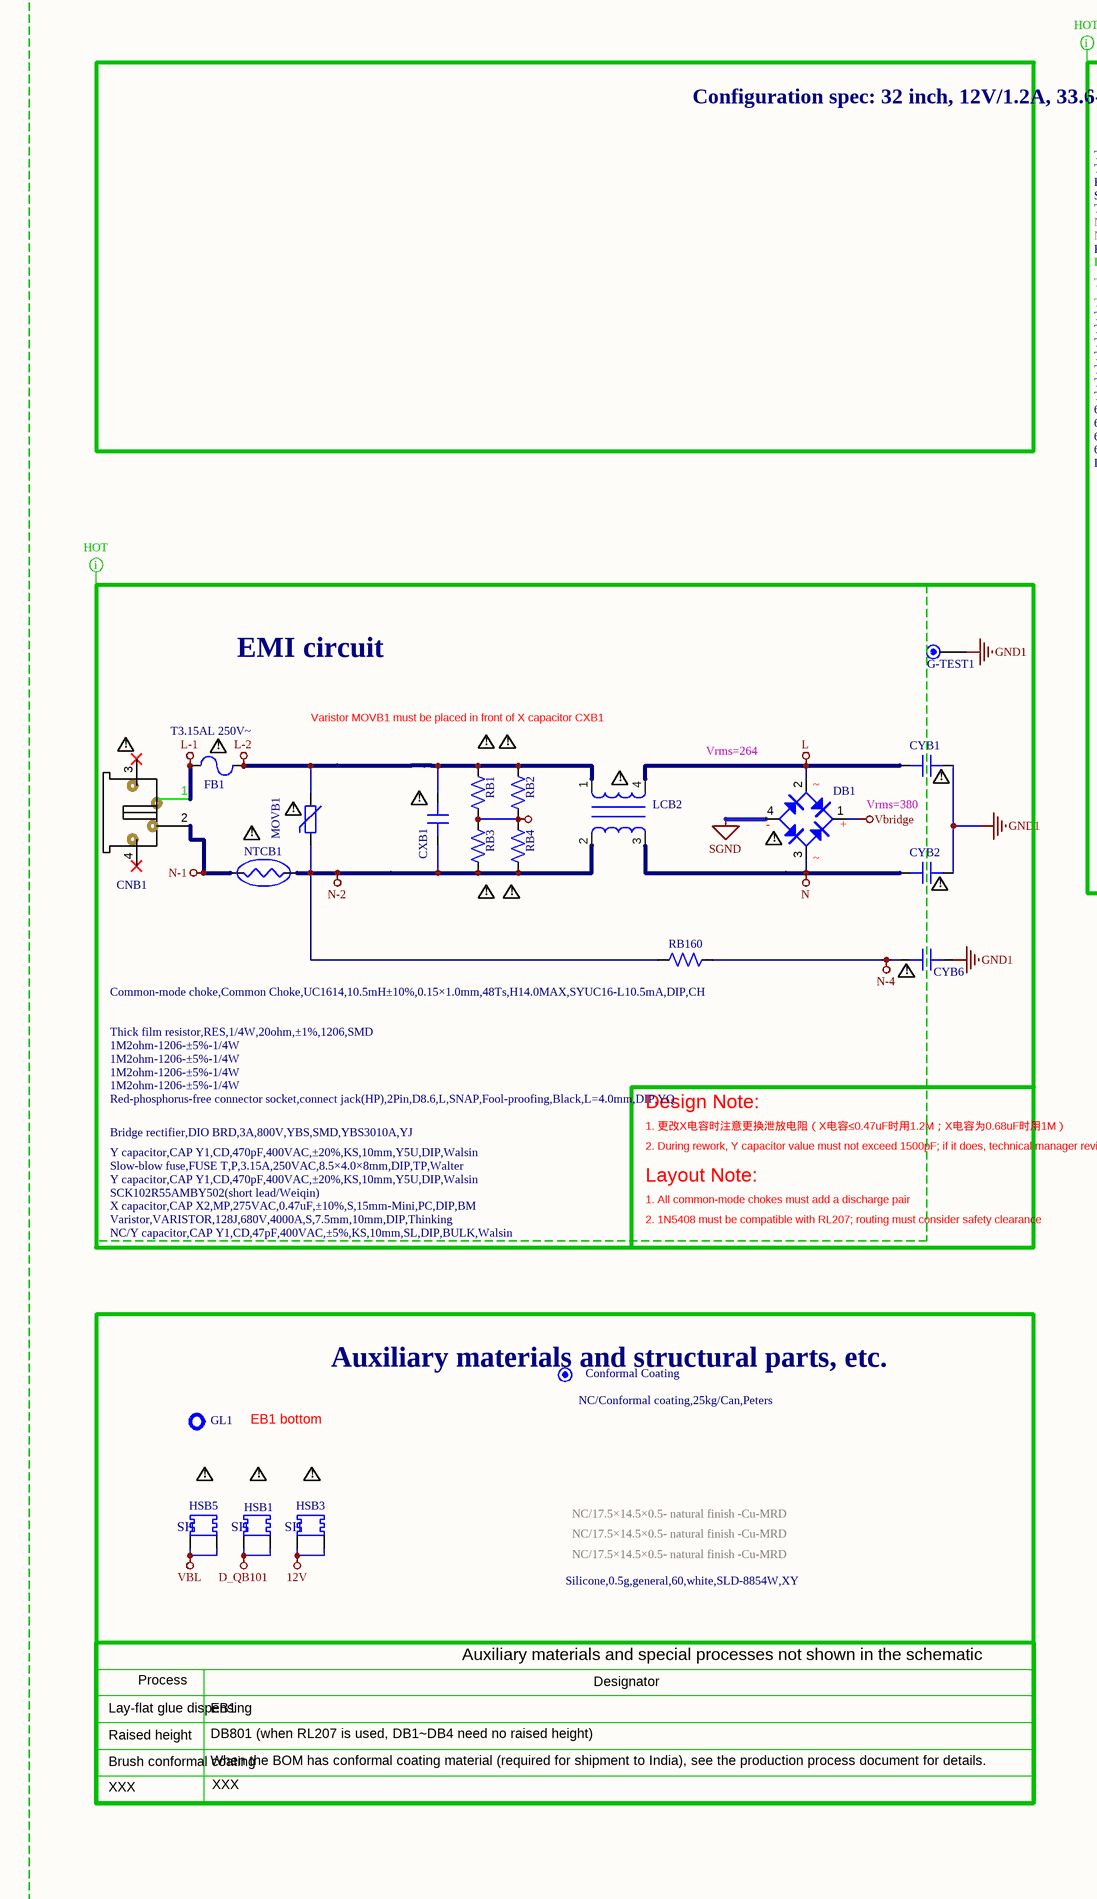
[diagram p0: MISC86383-5.SchDoc, left]
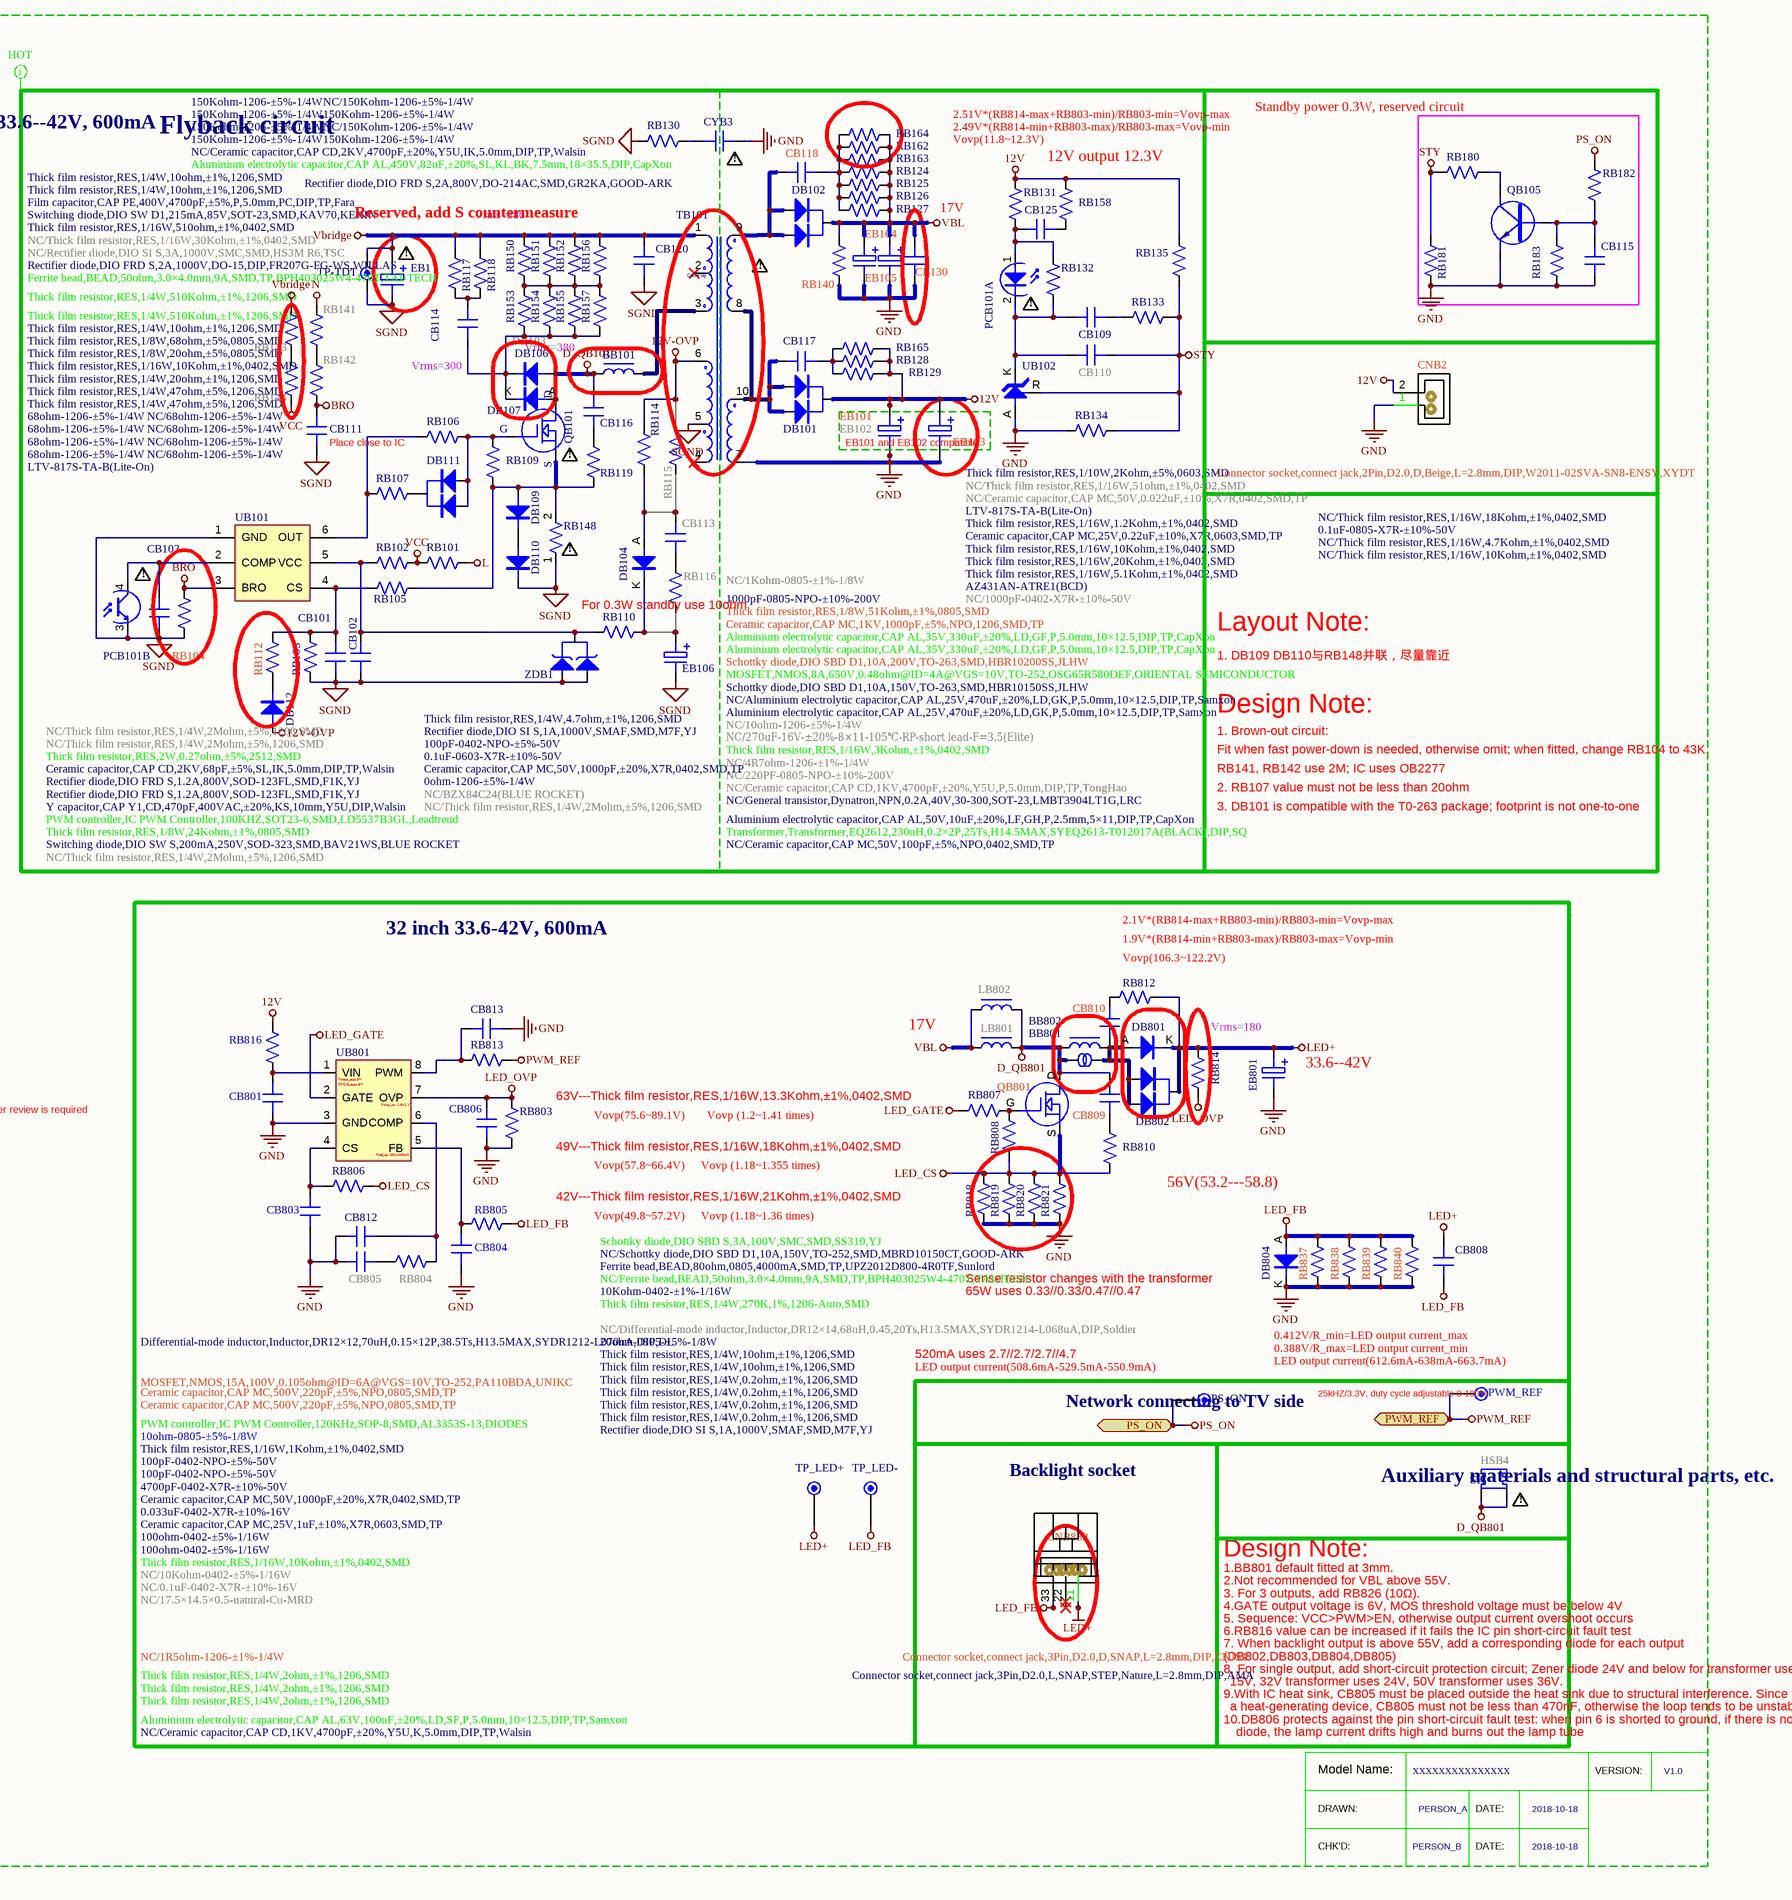
[diagram p1: MISC86383-5.SchDoc, right]
# Altium project MISC86383-33.PrjPCB (part 7 of 8)

## Sheet MISC86383-5.SchDoc: MISC86383
size A2

### Parts
BB101  Ferrite bead,BEAD,50ohm,3.0×4.0mm,9A,SMD,TP,BPH403025W4-470T,TAI-TECH  [L(4*3*2.55)-S]
BB801  Ferrite bead,BEAD,80ohm,0805,4000mA,SMD,TP,UPZ2012D800-4R0TF,Sunlord  [R0805]
BB802  NC/Ferrite bead,BEAD,50ohm,3.0×4.0mm,9A,SMD,TP,BPH403025W4-470T,TAI-TECH  [L(4*3*2.55)-S]
CB101  100pF-0402-NPO-±5%-50V  [C0402]
CB102  0.1uF-0603-X7R-±10%-50V  [C0603]
CB103  Ceramic capacitor,CAP MC,50V,1000pF,±20%,X7R,0402,SMD,TP  [C0402]
CB109  Ceramic capacitor,CAP MC,25V,0.22uF,±10%,X7R,0603,SMD,TP  [C0603]
CB110  NC/1000pF-0402-X7R-±10%-50V  [C0402]
CB111  NC/Ceramic capacitor,CAP MC,50V,100pF,±5%,NPO,0402,SMD,TP  [C0402]
CB113  NC/220PF-0805-NPO-±10%-200V  [C0805]
CB114  Film capacitor,CAP PE,400V,4700pF,±5%,P,5.0mm,PC,DIP,TP,Fara  [CAP8*2.5-V-5]
CB115  0.1uF-0805-X7R-±10%-50V  [C0805]
CB116  Ceramic capacitor,CAP CD,2KV,68pF,±5%,SL,IK,5.0mm,DIP,TP,Walsin  [CAP6.5*5-V-5-1]
CB117  1000pF-0805-NPO-±10%-200V  [C0805]
CB118  Ceramic capacitor,CAP MC,1KV,1000pF,±5%,NPO,1206,SMD,TP  [C1206]
CB120  NC/Ceramic capacitor,CAP CD,2KV,4700pF,±20%,Y5U,IK,5.0mm,DIP,TP,Walsin  [CAP10*4.5-V-5]
CB125  NC/Ceramic capacitor,CAP MC,50V,0.022uF,±10%,X7R,0402,SMD,TP  [C0402]
CB130  NC/Ceramic capacitor,CAP CD,1KV,4700pF,±20%,Y5U,P,5.0mm,DIP,TP,TongHao  [CAP9.8*4-V-5]
CB801  Ceramic capacitor,CAP MC,25V,1uF,±10%,X7R,0603,SMD,TP  [C0603]
CB803  100pF-0402-NPO-±5%-50V  [C0402]
CB804  4700pF-0402-X7R-±10%-50V  [C0402]
CB805  NC/0.1uF-0402-X7R-±10%-16V  [C0402]
CB806  Ceramic capacitor,CAP MC,50V,1000pF,±20%,X7R,0402,SMD,TP  [C0402]
CB808  NC/Ceramic capacitor,CAP CD,1KV,4700pF,±20%,Y5U,K,5.0mm,DIP,TP,Walsin  [CAP10*4.5-V-5]
CB809  Ceramic capacitor,CAP MC,500V,220pF,±5%,NPO,0805,SMD,TP  [C0805]
CB810  Ceramic capacitor,CAP MC,500V,220pF,±5%,NPO,0805,SMD,TP  [C0805]
CB812  0.033uF-0402-X7R-±10%-16V  [C0402]
CB813  100pF-0402-NPO-±5%-50V  [C0402]
CNB1  Red-phosphorus-free connector socket,connect jack(HP),2Pin,D8.6,L,SNAP,Fool-proofing,Black,L=4.0mm,DIP,YQ  [CON2-H8.6-1]
CNB2  Connector socket,connect jack,2Pin,D2.0,D,Beige,L=2.8mm,DIP,W2011-02SVA-SN8-ENSY,XYDT  [SIP2/2.0D-1]
CNB832  Connector socket,connect jack,3Pin,D2.0,D,SNAP,L=2.8mm,DIP,CNJST  [SIP3/2.0D-CP]
CNB833  Connector socket,connect jack,3Pin,D2.0,L,SNAP,STEP,Nature,L=2.8mm,DIP,AMA  [SIP3H/2.0D-3]
Conformal_Coating  NC/Conformal coating,25kg/Can,Peters  [Conformal Coating]
CXB1  X capacitor,CAP X2,MP,275VAC,0.47uF,±10%,S,15mm-Mini,PC,DIP,BM  [CAP18*8.5-V-15]
CYB1  Y capacitor,CAP Y1,CD,470pF,400VAC,±20%,KS,10mm,Y5U,DIP,Walsin  [CAP13*5-V-10-1]
CYB2  Y capacitor,CAP Y1,CD,470pF,400VAC,±20%,KS,10mm,Y5U,DIP,Walsin  [CAP13*5-V-10-1]
CYB3  Y capacitor,CAP Y1,CD,470pF,400VAC,±20%,KS,10mm,Y5U,DIP,Walsin  [CAP13*5-V-10-1]
CYB6  NC/Y capacitor,CAP Y1,CD,47pF,400VAC,±5%,KS,10mm,SL,DIP,BULK,Walsin  [CAP13*5-V-10-1]
DB1  Bridge rectifier,DIO BRD,3A,800V,YBS,SMD,YBS3010A,YJ  [B/YBS3010A]
DB101  Schottky diode,DIO SBD D1,10A,150V,TO-263,SMD,HBR10150SS,JLHW  [D2PAK3]
DB102  Schottky diode,DIO SBD D1,10A,200V,TO-263,SMD,HBR10200SS,JLHW  [D2PAK3]
DB103  NC/Rectifier diode,DIO SI S,3A,1000V,SMC,SMD,HS3M R6,TSC  [DIODE-SMC]
DB104  Rectifier diode,DIO SI S,1A,1000V,SMAF,SMD,M7F,YJ  [DIODE-S-2]
DB106  Rectifier diode,DIO FRD S,2A,1000V,DO-15,DIP,FR207G-FG-WS,WILLAS  [D2-H-15]
DB107  Rectifier diode,DIO FRD S,2A,800V,DO-214AC,SMD,GR2KA,GOOD-ARK  [DIODE-S-2]
DB109  Rectifier diode,DIO FRD S,1.2A,800V,SOD-123FL,SMD,F1K,YJ  [DIODE-S-14]
DB110  Rectifier diode,DIO FRD S,1.2A,800V,SOD-123FL,SMD,F1K,YJ  [DIODE-S-14]
DB111  Switching diode,DIO SW D1,215mA,85V,SOT-23,SMD,KAV70,KEXIN  [SO-23]
DB112  Switching diode,DIO SW S,200mA,250V,SOD-323,SMD,BAV21WS,BLUE ROCKET  [DIODE-S-12]
DB801  Schottky diode,DIO SBD S,3A,100V,SMC,SMD,SS310,YJ  [DIODE-SMC]
DB802  NC/Schottky diode,DIO SBD D1,10A,150V,TO-252,SMD,MBRD10150CT,GOOD-ARK  [TO-252]
DB804  Rectifier diode,DIO SI S,1A,1000V,SMAF,SMD,M7F,YJ  [DIODE-S-2]
EB1  Aluminium electrolytic capacitor,CAP AL,450V,82uF,±20%,SL,KL,BK,7.5mm,18×35.5,DIP,CapXon  [EC(18*36)-H7.5-1]
EB101  Aluminium electrolytic capacitor,CAP AL,25V,470uF,±20%,LD,GK,P,5.0mm,10×12.5,DIP,TP,Samxon  [EC(10*12.5)-V-5]
EB102  NC/270uF-16V-±20%-8×11-105℃-RP-short lead-F=3.5(Elite)  [EC(8*11)-V-3.5]
EB103  NC/Aluminium electrolytic capacitor,CAP AL,25V,470uF,±20%,LD,GK,P,5.0mm,10×12.5,DIP,TP,Samxon  [EC(10*12.5)-V-5]
EB104  Aluminium electrolytic capacitor,CAP AL,35V,330uF,±20%,LD,GF,P,5.0mm,10×12.5,DIP,TP,CapXon  [EC(10*12.5)-V-5]
EB105  Aluminium electrolytic capacitor,CAP AL,35V,330uF,±20%,LD,GF,P,5.0mm,10×12.5,DIP,TP,CapXon  [EC(10*12.5)-V-5]
EB106  Aluminium electrolytic capacitor,CAP AL,50V,10uF,±20%,LF,GH,P,2.5mm,5×11,DIP,TP,CapXon  [EC(5*11)-V-2.5]
EB801  Aluminium electrolytic capacitor,CAP AL,63V,100uF,±20%,LD,SF,P,5.0mm,10×12.5,DIP,TP,Samxon  [EC(10*12.5)-V-5]
FB1  Slow-blow fuse,FUSE T,P,3.15A,250VAC,8.5×4.0×8mm,DIP,TP,Walter  [FUSE8.5*4-V-5(T3.15AL 250V~)]
G-TEST1  TEST  [TP]  (value not drawn)
GL1  Silicone,0.5g,general,60,white,SLD-8854W,XY  [Silica gel-20]
HSB1  NC/17.5×14.5×0.5- natural finish -Cu-MRD  [HS038]
HSB3  NC/17.5×14.5×0.5- natural finish -Cu-MRD  [HS038]
HSB4  NC/17.5×14.5×0.5-natural-Cu-MRD  [HS038]
HSB5  NC/17.5×14.5×0.5- natural finish -Cu-MRD  [HS038]
LB801  Differential-mode inductor,Inductor,DR12×12,70uH,0.15×12P,38.5Ts,H13.5MAX,SYDR1212-L070uA,DIP,DL  [L/LC2/15*14.5-V7.5]
LB802  NC/Differential-mode inductor,Inductor,DR12×14,68uH,0.45,20Ts,H13.5MAX,SYDR1214-L068uA,DIP,Soldier  [L(13.5*15.5)-V-5]
LCB2  Common-mode choke,Common Choke,UC1614,10.5mH±10%,0.15×1.0mm,48Ts,H14.0MAX,SYUC16-L10.5mA,DIP,CH  [L/LC4/21*17-H-17*13]
MOVB1  Varistor,VARISTOR,128J,680V,4000A,S,7.5mm,10mm,DIP,Thinking  [VR(13*5)-V-7.5]
NTCB1  SCK102R55AMBY502(short lead/Weiqin)  [NTC(10*5)-V5]
PCB101  LTV-817S-TA-B(Lite-On)  [OC4-S-1]  (parts A,B of 2)
PS_ON  TEST  [TP_BL]  (value not drawn)
PWM_REF  NC/TEST  [TP_BL]  (value not drawn)
QB101  MOSFET,NMOS,8A,650V,0.48ohm@ID=4A@VGS=10V,TO-252,OSG65R580DEF,ORIENTAL SEMICONDUCTOR  [D2PAK3]
QB105  NC/General transistor,Dynatron,NPN,0.2A,40V,30-300,SOT-23,LMBT3904LT1G,LRC  [SOT-23]
QB801  MOSFET,NMOS,15A,100V,0.105ohm@ID=6A@VGS=10V,TO-252,PA110BDA,UNIKC  [TO-252-GDS]
RB1  1M2ohm-1206-±5%-1/4W  [R1206]
RB2  1M2ohm-1206-±5%-1/4W  [R1206]
RB3  1M2ohm-1206-±5%-1/4W  [R1206]
RB4  1M2ohm-1206-±5%-1/4W  [R1206]
RB101  Thick film resistor,RES,1/4W,510Kohm,±1%,1206,SMD  [R1206]
RB102  Thick film resistor,RES,1/4W,510Kohm,±1%,1206,SMD  [R1206]
RB103  Thick film resistor,RES,1/16W,3Kohm,±1%,0402,SMD  [R0402]
RB104  NC/Thick film resistor,RES,1/16W,30Kohm,±1%,0402,SMD  [R0402]
RB105  Thick film resistor,RES,1/16W,510ohm,±1%,0402,SMD  [R0402]
RB106  Thick film resistor,RES,1/8W,68ohm,±5%,0805,SMD  [R0805]
RB107  Thick film resistor,RES,1/8W,20ohm,±5%,0805,SMD  [R0805]
RB109  Thick film resistor,RES,1/16W,10Kohm,±1%,0402,SMD  [R0402]
RB110  0ohm-1206-±5%-1/4W  [R1206]
RB112  Thick film resistor,RES,1/8W,24Kohm,±1%,0805,SMD  [R0805]
RB114  Thick film resistor,RES,1/4W,4.7ohm,±1%,1206,SMD  [R1206]
RB115  NC/4R7ohm-1206-±1%-1/4W  [R1206]
RB116  NC/10ohm-1206-±5%-1/4W  [R1206]
RB117  Thick film resistor,RES,1/4W,10ohm,±1%,1206,SMD  [R1206]
RB118  Thick film resistor,RES,1/4W,10ohm,±1%,1206,SMD  [R1206]
RB119  Thick film resistor,RES,1/4W,10ohm,±1%,1206,SMD  [R1206]
RB124  68ohm-1206-±5%-1/4W  [R1206]
RB125  68ohm-1206-±5%-1/4W  [R1206]
RB126  68ohm-1206-±5%-1/4W  [R1206]
RB127  68ohm-1206-±5%-1/4W  [R1206]
RB128  Thick film resistor,RES,1/4W,47ohm,±5%,1206,SMD  [R1206]
RB129  Thick film resistor,RES,1/4W,47ohm,±5%,1206,SMD  [R1206]
RB130  Thick film resistor,RES,1/4W,20ohm,±1%,1206,SMD  [R1206]
RB131  Thick film resistor,RES,1/10W,2Kohm,±5%,0603,SMD  [R0603]
RB132  Thick film resistor,RES,1/16W,1.2Kohm,±1%,0402,SMD  [R0402]
RB133  Thick film resistor,RES,1/16W,10Kohm,±1%,0402,SMD  [R0402]
RB134  Thick film resistor,RES,1/16W,5.1Kohm,±1%,0402,SMD  [R0402]
RB135  Thick film resistor,RES,1/16W,20Kohm,±1%,0402,SMD  [R0402]
RB140  Thick film resistor,RES,1/8W,51Kohm,±1%,0805,SMD  [R0805]
RB141  NC/Thick film resistor,RES,1/4W,2Mohm,±5%,1206,SMD  [R1206]
RB142  NC/Thick film resistor,RES,1/4W,2Mohm,±5%,1206,SMD  [R1206]
RB143  NC/Thick film resistor,RES,1/4W,2Mohm,±5%,1206,SMD  [R1206]
RB144  NC/Thick film resistor,RES,1/4W,2Mohm,±5%,1206,SMD  [R1206]
RB148  Thick film resistor,RES,2W,0.27ohm,±5%,2512,SMD  [R2512-1]
RB150  150Kohm-1206-±5%-1/4W  [R1206]
RB151  150Kohm-1206-±5%-1/4W  [R1206]
RB152  150Kohm-1206-±5%-1/4W  [R1206]
RB153  150Kohm-1206-±5%-1/4W  [R1206]
RB154  150Kohm-1206-±5%-1/4W  [R1206]
RB155  150Kohm-1206-±5%-1/4W  [R1206]
RB156  NC/150Kohm-1206-±5%-1/4W  [R1206]
RB157  NC/150Kohm-1206-±5%-1/4W  [R1206]
RB158  NC/Thick film resistor,RES,1/16W,51ohm,±1%,0402,SMD  [R0402]
RB160  Thick film resistor,RES,1/4W,20ohm,±1%,1206,SMD  [R1206]
RB162  NC/68ohm-1206-±5%-1/4W  [R1206]
RB163  NC/68ohm-1206-±5%-1/4W  [R1206]
RB164  NC/68ohm-1206-±5%-1/4W  [R1206]
RB165  NC/68ohm-1206-±5%-1/4W  [R1206]
RB180  NC/Thick film resistor,RES,1/16W,18Kohm,±1%,0402,SMD  [R0402]
RB181  NC/1Kohm-0805-±1%-1/8W  [R0805]
RB182  NC/Thick film resistor,RES,1/16W,4.7Kohm,±1%,0402,SMD  [R0402]
RB183  NC/Thick film resistor,RES,1/16W,10Kohm,±1%,0402,SMD  [R0402]
RB803  Thick film resistor,RES,1/16W,10Kohm,±1%,0402,SMD  [R0402]
RB804  NC/10Kohm-0402-±5%-1/16W  [R0402]
RB805  100ohm-0402-±5%-1/16W  [R0402]
RB806  Thick film resistor,RES,1/16W,1Kohm,±1%,0402,SMD  [R0402]
RB807  20ohm-0805-±5%-1/8W  [R0805]
RB808  10Kohm-0402-±1%-1/16W  [R0402]
RB810  Thick film resistor,RES,1/4W,10ohm,±1%,1206,SMD  [R1206]
RB812  Thick film resistor,RES,1/4W,10ohm,±1%,1206,SMD  [R1206]
RB813  100ohm-0402-±5%-1/16W  [R0402]
RB814  Thick film resistor,RES,1/4W,270K,1%,1206-Auto,SMD  [R1206]
RB816  10ohm-0805-±5%-1/8W  [R0805]
RB818  Thick film resistor,RES,1/4W,0.2ohm,±1%,1206,SMD  [R1206]
RB819  Thick film resistor,RES,1/4W,0.2ohm,±1%,1206,SMD  [R1206]
RB820  Thick film resistor,RES,1/4W,0.2ohm,±1%,1206,SMD  [R1206]
RB821  Thick film resistor,RES,1/4W,0.2ohm,±1%,1206,SMD  [R1206]
RB837  Thick film resistor,RES,1/4W,2ohm,±1%,1206,SMD  [R1206]
RB838  Thick film resistor,RES,1/4W,2ohm,±1%,1206,SMD  [R1206]
RB839  Thick film resistor,RES,1/4W,2ohm,±1%,1206,SMD  [R1206]
RB840  NC/1R5ohm-1206-±1%-1/4W  [R1206]
TB101  Transformer,Transformer,EQ2612,230uH,0.2×2P,25Ts,H14.5MAX,SYEQ2613-T012017A(BLACK),DIP,SQ  [T/EQ2612*10]
TP-TDT  NC/  [TP-TDT]  (value not drawn)
TP_LED+  NC/  [TP]  (value not drawn)
TP_LED-  NC/  [TP]  (value not drawn)
UB101  PWM controller,IC PWM Controller,100KHZ,SOT23-6,SMD,LD5537B3GL,Leadtrend  [SOT-26]
UB102  AZ431AN-ATRE1(BCD)  [SOT-23-RAK]
UB801  PWM controller,IC PWM Controller,120KHz,SOP-8,SMD,AL3353S-13,DIODES  [SO-8A]
ZDB1  NC/BZX84C24(BLUE ROCKET)  [SO-23]

### Blocks framed on the sheet
Vrms=380: DB103 DB106 DB107
EB101 and EB102 compatible: EB101-EB103
EMI circuit: CNB1 CXB1 CYB1 CYB2 CYB6 DB1 FB1 G-TEST1 LCB2 MOVB1 NTCB1 RB1-RB4 RB160
Auxiliary materials and structural parts, etc.: Conformal_Coating GL1 HSB1 HSB3 HSB5

### Ports
PS_ON, PWM_REF

### Nets
12V: CNB2.2 DB101.2 EB101.1 EB102.1 EB103.1 HSB3.1 HSB3.2 RB128.2 RB129.2 RB131.2 RB135.1 RB158.2 RB165.2 RB816.1
12V-OVP: DB112.A RB114.2 RB115.2 TB101.6
BRO: CB111.1 RB104.2 RB142.1 UB101.3(BRO)
D_QB101: BB101.1 CB116.2 DB103.A DB106.A DB107.A HSB1.1 HSB1.2 QB101.2(D)
D_QB801: BB801.1 BB802.1 CB809.2 HSB4.1 HSB4.2 LB801.2 LB802.2 QB801.D
GND: CB115.2 CB130.1 CB801.1 CB803.2 CB804.2 CB805.1 CB806.2 CB812.1 CB813.1 CNB2.1 CYB3.2 DB804.K EB101.2 EB102.2 EB103.2 EB104.2 EB105.2 EB801.2 QB105.E RB134.1 RB140.2 RB181.1 RB183.2 RB803.1 RB818.2 RB819.2 RB820.2 RB821.2 RB837.1 RB838.1 RB839.2 RB840.1 TB101.7 UB102.A UB801.3(GND)
GND1: CYB1.2 CYB2.2 CYB6.2 G-TEST1.1
L: CYB1.1 DB1.2 LCB2.4 RB101.1
L-1: CNB1.1 FB1.1
L-2: CXB1.1 FB1.2 LCB2.1 MOVB1.1 RB1.1 RB2.1
L-N: RB1.2 RB2.2 RB3.1 RB4.1
LED+: CB808.2 CNB832.1 CNB833.1 DB801.K DB802.2 EB801.1 RB812.2 RB814.1 TP_LED+.1
LED_CS: QB801.S RB806.2 RB808.1 RB810.2 RB818.1 RB819.1 RB820.1 RB821.1
LED_FB: CB808.1 CNB832.3 CNB833.3 DB804.A RB805.2 RB837.2 RB838.2 RB839.1 RB840.2 TP_LED-.1
LED_GATE: RB807.1 UB801.2(GATE)
LED_OVP: CB806.1 RB803.2 RB814.2 UB801.7(OVP)
N: CYB2.1 DB1.3 LCB2.3 RB141.2
N-1: CNB1.2 NTCB1.2
N-2: CXB1.2 LCB2.2 MOVB1.2 NTCB1.1 RB3.2 RB4.2 RB160.1
N-4: CYB6.1 RB160.2
PS_ON: PS_ON.1 RB182.2 ; port PS_ON
PWM_REF: PWM_REF.1 RB813.2 ; port PWM_REF
SGND: CB101.2 CB102.2 CB103.2 CB111.2 CB120.1 DB1.4 DB110.K EB1.2 EB106.2 PCB101.3 RB103.1 RB104.1 RB130.1 RB148.1 TB101.5 TP-TDT.2 UB101.1(GND) ZDB1.1 ZDB1.3
STY: CB110.2 RB133.1 RB134.2 RB135.2 RB180.2 RB181.2 UB102.R
VBL: CB130.2 DB102.2 EB104.1 EB105.1 HSB5.1 HSB5.2 LB801.1 LB802.1 RB124.2 RB125.2 RB126.2 RB127.2 RB140.1 RB162.2 RB163.2 RB164.2
Vbridge: CB120.2 DB1.1 EB1.1 RB117.2 RB118.2 RB143.2 RB150.2 RB151.2 RB152.2 RB156.2 TB101.1 TP-TDT.1
VCC: RB101.2 RB102.1 RB144.1
NetBB101_2: BB101.2 TB101.3
NetBB801_2: BB801.2 BB802.2 CB810.1 DB801.A DB802.1 DB802.3
NetCB101_1: CB101.1 RB103.2 RB105.1 RB112.1 UB101.4(CS)
NetCB102_1: CB102.1 RB102.2 RB110.1 UB101.5(VCC) ZDB1.2
NetCB103_1: CB103.1 PCB101.4 UB101.2(COMP)
NetCB109_1: CB109.1 CB110.1 PCB101.2 RB132.1 UB102.K
NetCB109_2: CB109.2 RB133.2
NetCB113_1: CB113.1 DB104.A RB114.1 RB115.1
NetCB113_2: CB113.2 RB116.1
NetCB114_1: CB114.1 RB117.1 RB118.1
NetCB114_2: CB114.2 DB103.K DB106.K DB107.K RB153.1 RB154.1 RB155.1 RB157.1
NetCB115_1: CB115.1 QB105.B RB182.1 RB183.1
NetCB116_1: CB116.1 RB119.2
NetCB117_1: CB117.1 DB101.1 DB101.3 TB101.8 TB101.10
NetCB117_2: CB117.2 RB128.1 RB129.1 RB165.1
NetCB118_1: CB118.1 DB102.1 DB102.3 TB101.9
NetCB118_2: CB118.2 RB124.1 RB125.1 RB126.1 RB127.1 RB162.1 RB163.1 RB164.1
NetCB125_1: CB125.1 PCB101.1 RB131.1 RB132.2
NetCB125_2: CB125.2 RB158.1
NetCB801_2: CB801.2 RB816.2 UB801.1(VIN)
NetCB803_1: CB803.1 RB806.1 UB801.4(CS)
NetCB804_1: CB804.1 RB805.1 UB801.5(FB)
NetCB805_2: CB805.2 RB804.1
NetCB809_1: CB809.1 RB810.1
NetCB810_2: CB810.2 RB812.1
NetCB812_2: CB812.2 RB804.2 UB801.6(COMP)
NetCB813_2: CB813.2 RB813.1 UB801.8(PWM)
NetCYB3_1: CYB3.1 RB130.2
NetDB104_K: DB104.K EB106.1 RB110.2 RB116.2
NetDB109_A: DB109.A QB101.3(S) RB105.2 RB109.1 RB119.1 RB148.2
NetDB109_K: DB109.K DB110.A
NetDB111_1: DB111.1 DB111.3 QB101.1(G) RB106.2 RB109.2
NetDB111_2: DB111.2 RB107.2
NetDB112_K: DB112.K RB112.2
NetQB105_C: QB105.C RB180.1
NetQB801_G: QB801.G RB807.2 RB808.2
NetRB106_1: RB106.1 RB107.1 UB101.6(OUT)
NetRB141_1: RB141.1 RB142.2
NetRB143_1: RB143.1 RB144.2
NetRB150_1: RB150.1 RB151.1 RB152.1 RB153.2 RB154.2 RB155.2 RB156.1 RB157.2

Not connected (* = marked no-connect by the designer): CNB1 3* 4*; CNB832 2*; CNB833 2*; TB101 2* 4*

### Layout directives
net class HOT: 12V, 12V-OVP, BRO, D_QB101, D_QB801, GND, GND1, L, L-1, L-2, L-N, LED+, LED_CS, LED_FB, LED_GATE, LED_OVP, N, N-1, N-2, N-4, PS_ON, PWM_REF, SGND, STY, VBL, Vbridge, VCC
net class POWER: 12V, 12V-OVP, BRO, D_QB101, D_QB801, GND, GND1, L, L-1, L-2, L-N, LED+, LED_CS, LED_FB, LED_GATE, LED_OVP, N, N-1, N-2, N-4, PS_ON, PWM_REF, SGND, STY, VBL, Vbridge, VCC

### Notes on the sheet
- 2.51V*(RB814-max+RB803-min)/RB803-min=Vovp-max
- Standby power 0.3W, reserved circuit
- Configuration spec: 32 inch, 12V/1.2A, 33.6--42V, 600mA
- Flyback circuit
- (near CYB3) !
- 2.49V*(RB814-min+RB803-max)/RB803-max=Vovp-min
- Vovp(11.8~12.3V)
- (near RB158) 12V output 12.3V
- Reserved, add S countermeasure
- (near EB1) !
- Vrms=380
- 17V
- !
- (near CB114) Vrms=300
- Place close to IC
- (near RB148) !
- (near RB116) For 0.3W standby use 10ohm
- 1. DB109 DB110与RB148并联，尽量靠近
- Layout Note:
- (near CNB1) !
- (near FB1) !
- Varistor MOVB1 must be placed in front of X capacitor CXB1
- (near DB1) Vrms=264
- 1. Brown-out circuit:
- Fit when fast power-down is needed, otherwise omit; when fitted, change RB104 to 43K,
- Design Note:
- (near NTCB1) !
- (near MOVB1) !
- (near CXB1) !
- (near LCB2) !
- (near DB1) !
- (near CYB1) !
- RB141, RB142 use 2M; IC uses OB2277
- 2. RB107 value must not be less than 20ohm
- 3. DB101 is compatible with the T0-263 package; footprint is not one-to-one
- (near CYB2) !
- (near CYB6) !
- 32 inch 33.6-42V, 600mA
- 2.1V*(RB814-max+RB803-min)/RB803-min=Vovp-max
- 1.9V*(RB814-min+RB803-max)/RB803-max=Vovp-min
- Vovp(106.3~122.2V)
- Vrms=180
- (near EB801) 33.6--42V
- 1. 更改X电容时注意更换泄放电阻（X电容≤0.47uF时用1.2M；X电容为0.68uF时用1M）
- 2. During rework, Y capacitor value must not exceed 1500pF; if it does, technical manager review is required
- 63V---Thick film resistor,RES,1/16W,13.3Kohm,±1%,0402,SMD
- Vovp(75.6~89.1V)
- Vovp (1.2~1.41 times)
- 1. All common-mode chokes must add a discharge pair
- 2. 1N5408 must be compatible with RL207; routing must consider safety clearance
- 49V---Thick film resistor,RES,1/16W,18Kohm,±1%,0402,SMD
- 42V---Thick film resistor,RES,1/16W,21Kohm,±1%,0402,SMD
- Vovp(57.8~66.4V)
- Vovp (1.18~1.355 times)
- 56V(53.2---58.8)
- Vovp(49.8~57.2V)
- Vovp (1.18~1.36 times)
- Sense resistor changes with the transformer
- 65W uses 0.33//0.33/0.47//0.47
- EB1 bottom
- 520mA uses 2.7//2.7/2.7//4.7
- (near PS_ON) LED output current(508.6mA-529.5mA-550.9mA)
- 0.412V/R_min=LED output current_max
- (near PWM_REF) 0.388V/R_max=LED output current_min
- (near PWM_REF) LED output current(612.6mA-638mA-663.7mA)
- Network connecting to TV side
- (near PWM_REF) 25kHZ/3.3V, duty cycle adjustable 0-100%
- (near TP_LED-) Backlight socket
- Auxiliary materials and structural parts, etc.
- (near HSB4) !
- 1.BB801 default fitted at 3mm.
- Process
- Auxiliary materials and special processes not shown in the schematic
- Designator
- 6.RB816 value can be increased if it fails the IC pin short-circuit fault test
- 3. For 3 outputs, add RB826 (10Ω).
- 2.Not recommended for VBL above 55V.
- 4.GATE output voltage is 6V, MOS threshold voltage must be below 4V
- 5. Sequence: VCC>PWM>EN, otherwise output current overshoot occurs
- Lay-flat glue dispensing
- Raised height
- Brush conformal coating
- EB1
- DB801 (when RL207 is used, DB1~DB4 need no raised height)
- When the BOM has conformal coating material (required for shipment to India), see the production process document for details.
- 8. For single output, add short-circuit protection circuit; Zener diode 24V and below for transformer use
- 7. When backlight output is above 55V, add a corresponding diode for each output
- (DB802,DB803,DB804,DB805)
- 9.With IC heat sink, CB805 must be placed outside the heat sink due to structural interference. Since the IC is
- 15V, 32V transformer uses 24V, 50V transformer uses 36V.
- XXX
- 10.DB806 protects against the pin short-circuit fault test: when pin 6 is shorted to ground, if there is no
- a heat-generating device, CB805 must not be less than 470nF, otherwise the loop tends to be unstable
- diode, the lamp current drifts high and burns out the lamp tube
- Model Name:
- DRAWN:
- XXXXXXXXXXXXXXX
- PERSON_A
- DATE:
- 2018-10-18
- VERSION:
- V1.0
- CHK'D:
- PERSON_B
- Title
- Size:
- Date:
- A4
- Number:
- Time:
- Revision:
- Sheet
- of
- File: